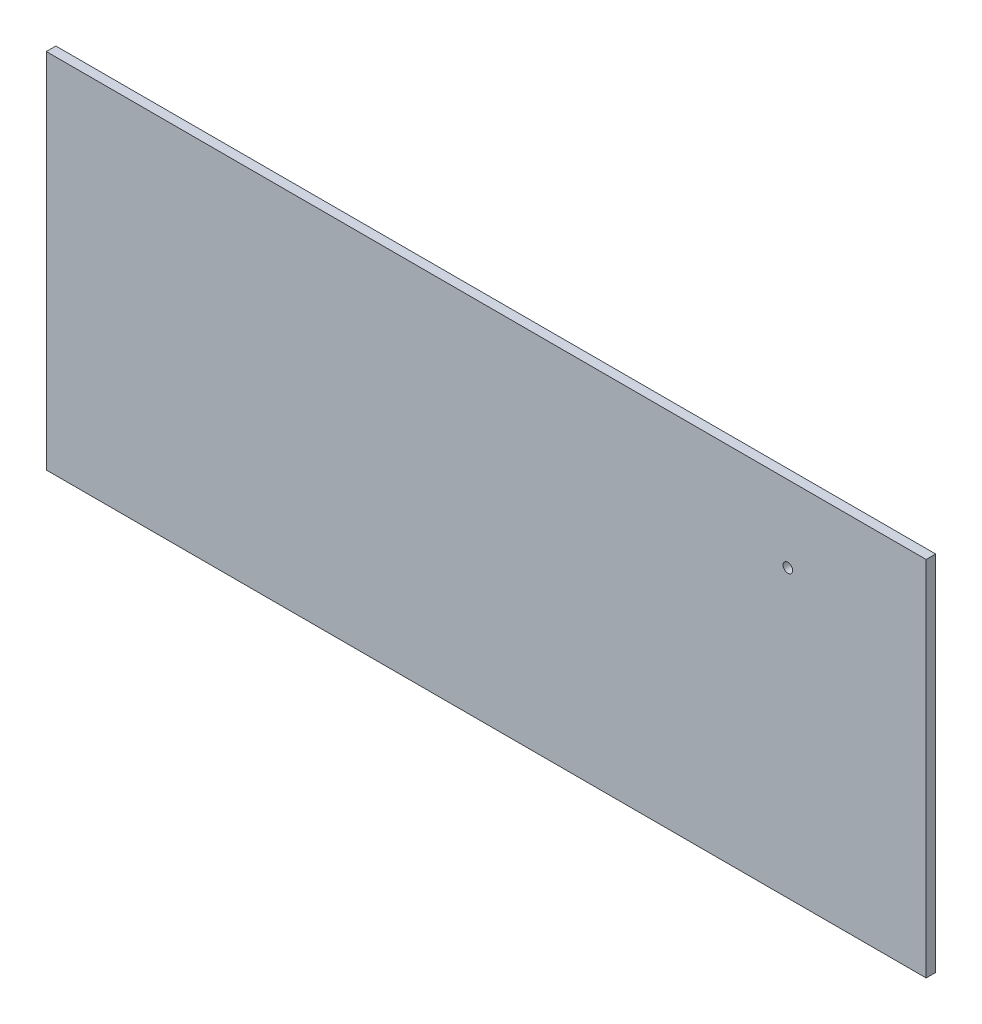
from build123d import *

# Parameters (mm, degrees)
SKETCH1_W           = 1845
SKETCH1_H           = 760
SKETCH1_R           = 10
BOSS_EXTRUDE1_DEPTH = 20


with BuildPart() as part:
    # Sketch1 → Boss-Extrude1 (new body)
    with BuildSketch(Plane.XY):
        with Locations((922.5, 380)):
            Rectangle(SKETCH1_W, SKETCH1_H)
        with Locations((1555, 600)):
            Circle(SKETCH1_R, mode=Mode.SUBTRACT)
    extrude(amount=BOSS_EXTRUDE1_DEPTH)


solid = part.part
